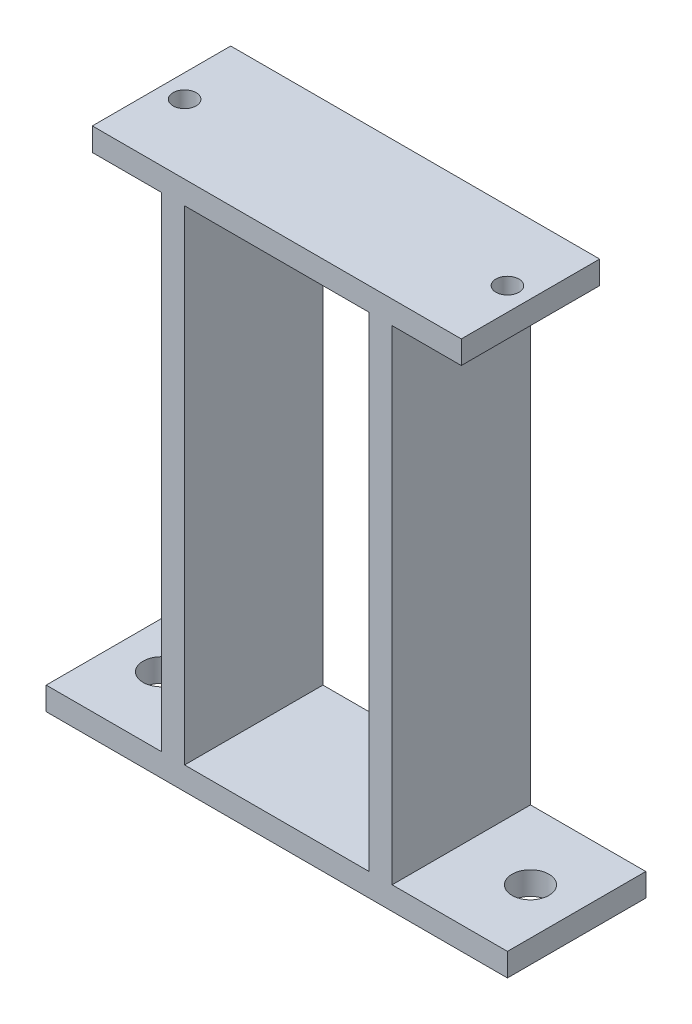
SolidWorks part; units mm, degrees
ref_plane "Front Plane" through (0, 0, 0) normal (0, 0, 1) x (1, 0, 0)
ref_plane "Top Plane" through (0, 0, 0) normal (0, 1, 0) x (1, 0, 0)
ref_plane "Right Plane" through (0, 0, 0) normal (1, 0, 0) x (0, 0, -1)
sketch "Sketch1" plane through (0, 0, 0) normal (0, 0, 1) x (1, 0, 0)
  line L0 (0, 0) -> (100, 0)
  line L1 (100, 0) -> (100, 5)
  line L2 (100, 5) -> (75, 5)
  line L3 (75, 5) -> (75, 110)
  line L4 (75, 110) -> (90, 110)
  line L5 (90, 110) -> (90, 115)
  line L6 (90, 115) -> (10, 115)
  line L7 (10, 115) -> (10, 110)
  line L8 (10, 110) -> (25, 110)
  line L9 (25, 110) -> (25, 5)
  line L10 (25, 5) -> (0, 5)
  line L11 (0, 5) -> (0, 0)
  line L13 (30, 110) -> (70, 110)
  line L14 (30, 110) -> (30, 5)
  line L15 (30, 5) -> (70, 5)
  line L16 (70, 110) -> (70, 5)
  dimension "D1" = 80
  dimension "D2" = 115
  dimension "D3" = 5
  dimension "D4" = 5
  dimension "D5" = 5
  dimension "D6" = 5
  dimension "D7" = 100
  dimension "D8" = 50
  dimension "D9" = 15
  dimension "D10" = 25
  dimension "D11" = 5
  dimension "D12" = 5
  dimension "D13" = 5
extrude "Boss-Extrude1" add sketch "Sketch1" along normal blind 30
sketch "Sketch2" plane through (0, 5, 0) normal (0, 1, 0) x (1, 0, 0)
  line L0 (100, -30) -> (100, 0) construction
  line L1 (0, -30) -> (0, 0) construction
  circle A0 centre (90, -15) radius 4
  circle A1 centre (10, -15) radius 4
  dimension "D1" = 8
  dimension "D2" = 10
  dimension "D3" = 8
  dimension "D4" = 10
extrude "Cut-Extrude1" cut sketch "Sketch2" against normal through all
sketch "Sketch3" plane through (0, 115, 0) normal (0, 1, 0) x (1, 0, 0)
  line L0 (10, -30) -> (10, 0) construction
  line L1 (90, -30) -> (90, 0) construction
  circle A0 centre (15, -15) radius 2.5
  circle A1 centre (85, -15) radius 2.5
  dimension "D1" = 5
  dimension "D2" = 5
  dimension "D3" = 5
  dimension "D4" = 5
extrude "Cut-Extrude2" cut sketch "Sketch3" against normal blind 10
